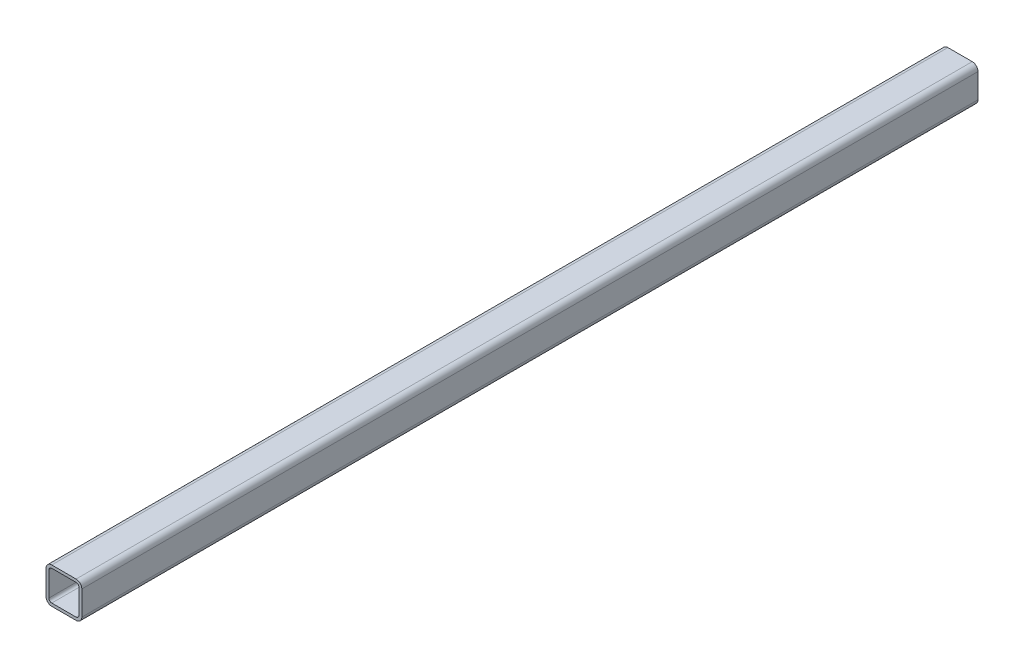
from build123d import *

# Parameters (mm, degrees)
BOSS_EXTRUDE1_DEPTH = 625


with BuildPart() as part:
    # Sketch1 → Boss-Extrude1 (new, symmetric)
    with BuildSketch(Plane.XY):
        with BuildLine():
            Line((-17, -25), (17, -25))
            ThreePointArc((17, -25), (22.656854249, -22.656854249), (25, -17))
            Line((25, -17), (25, 17))
            ThreePointArc((25, 17), (22.656854249, 22.656854249), (17, 25))
            Line((17, 25), (-17, 25))
            ThreePointArc((-17, 25), (-22.656854249, 22.656854249), (-25, 17))
            Line((-25, 17), (-25, -17))
            ThreePointArc((-25, -17), (-22.656854249, -22.656854249), (-17, -25))
        make_face()
        with BuildLine():
            Line((-17, 21), (17, 21))
            ThreePointArc((17, 21), (19.828427125, 19.828427125), (21, 17))
            Line((21, 17), (21, -17))
            ThreePointArc((21, -17), (19.828427125, -19.828427125), (17, -21))
            Line((17, -21), (-17, -21))
            ThreePointArc((-17, -21), (-19.828427125, -19.828427125), (-21, -17))
            Line((-21, -17), (-21, 17))
            ThreePointArc((-21, 17), (-19.828427125, 19.828427125), (-17, 21))
        make_face(mode=Mode.SUBTRACT)
    extrude(amount=BOSS_EXTRUDE1_DEPTH, both=True)


solid = part.part
